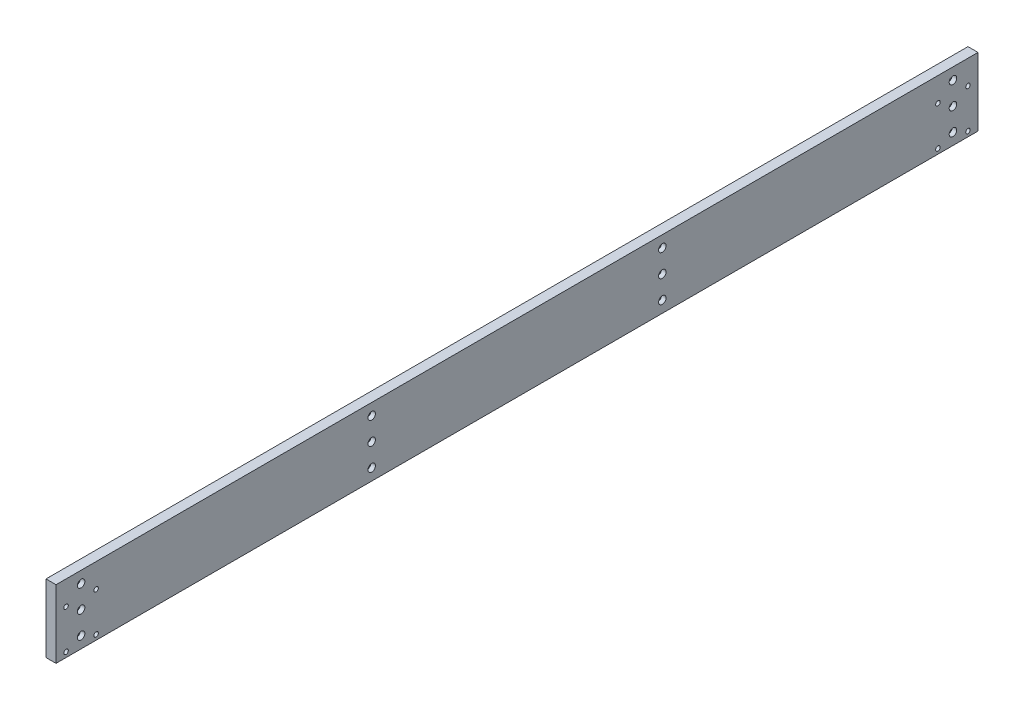
SolidWorks part; units mm, degrees
ref_plane "前视基准面" through (0, 0, 0) normal (0, 0, 1) x (1, 0, 0)
ref_plane "上视基准面" through (0, 0, 0) normal (0, 1, 0) x (1, 0, 0)
ref_plane "右视基准面" through (0, 0, 0) normal (1, 0, 0) x (0, 0, -1)
sketch "草图2" plane through (0, 0, 0) normal (1, 0, 0) x (0, 0, -1)
  line L1 (-920, 68) -> (920, 68)
  line L2 (-920, 68) -> (-920, -68)
  line L3 (-920, -68) -> (920, -68)
  line L4 (920, 68) -> (920, -68)
  line L5 (-920, 68) -> (920, -68) construction
  line L6 (-920, -68) -> (920, 68) construction
  point P0 (0, 0)
  dimension "D1" = 1840
  dimension "D2" = 136
extrude "凸台-拉伸2" add sketch "草图2" along normal blind 20
hole_wizard "打孔尺寸(%根据)内六角圆柱头螺钉的类型2" positions "草图3" profile "草图4" counterbore size "M8" standard "GB" end condition through all
sketch "草图3" plane through (20, 0, 0) normal (1, 0, 0) x (0, 0, -1)
  line L0 (-920, 0) -> (-645.5835, 0) construction
  line L1 (-920, 68) -> (-920, -68) construction
  point P0 (-870, 45)
  point P2 (-870, -45)
  point P11 (-870, 0)
  dimension "D1" = 90
  dimension "D2" = 50
sketch "草图4" plane through (20, 45, 870) normal (0, 1, 0) x (0, 0, -1)
  line L0 (0, 0) -> (0, 20)
  line L1 (0, 20) -> (4.5, 20)
  line L3 (4.5, 20) -> (4.5, 9)
  line L4 (4.5, 9) -> (7.5, 9)
  line L5 (7.5, 9) -> (7.5, 0)
  line L7 (7.5, 0) -> (0, 0)
  line L11 (0, -6.35) -> (0, 107.95) construction
  dimension "通孔孔直径" = 9
  dimension "通孔孔深度" = 20
  dimension "柱形沉头孔直径" = 15
  dimension "柱形沉头孔深度" = 9
pattern_linear "阵列(线性)1" count 4 spacing 580 along (0, 0, -1) of "打孔尺寸(%根据)内六角圆柱头螺钉的类型2"
hole_wizard "打孔尺寸(%根据)内六角圆柱头螺钉的类型2" positions "草图5" profile "草图6" counterbore size "M8" standard "GB" end condition through all
sketch "草图5" plane through (0, 0, 0) normal (-1, 0, 0) x (0, 0, 1)
  line L0 (0, 0) -> (0, 318.6159) construction
  line L1 (-920, 68) -> (920, 68) construction
  line L2 (-920, -68) -> (-920, 68) construction
  point P0 (-900, 20)
  point P2 (-840, 20)
  point P4 (-900, -58)
  point P6 (-840, -58)
  point P8 (840, 20)
  point P10 (900, 20)
  point P14 (840, -58)
  point P16 (900, -58)
  dimension "D1" = 48
  dimension "D2" = 78
  dimension "D3" = 60
  dimension "D4" = 20
sketch "草图6" plane through (0, 20, -900) normal (0, 1, 0) x (0, 0, 1)
  line L0 (0, 0) -> (0, 20)
  line L1 (0, 20) -> (4.5, 20)
  line L3 (4.5, 20) -> (4.5, 9)
  line L4 (7.5, 9) -> (4.5, 9)
  line L5 (7.5, 9) -> (7.5, 0.025)
  line L6 (7.5, 0.025) -> (7.525, 0)
  line L7 (7.525, 0) -> (0, 0)
  line L8 (-7.5, 0.025) -> (-7.525, 0) construction
  line L11 (0, -6.35) -> (0, 107.95) construction
  dimension "通孔孔直径" = 9
  dimension "通孔孔深度" = 20
  dimension "柱形沉头孔直径" = 15
  dimension "柱形沉头孔深度" = 9
  dimension "近端锥形沉头孔直径" = 15.05
  dimension "近端锥形沉头孔角度" = 90
